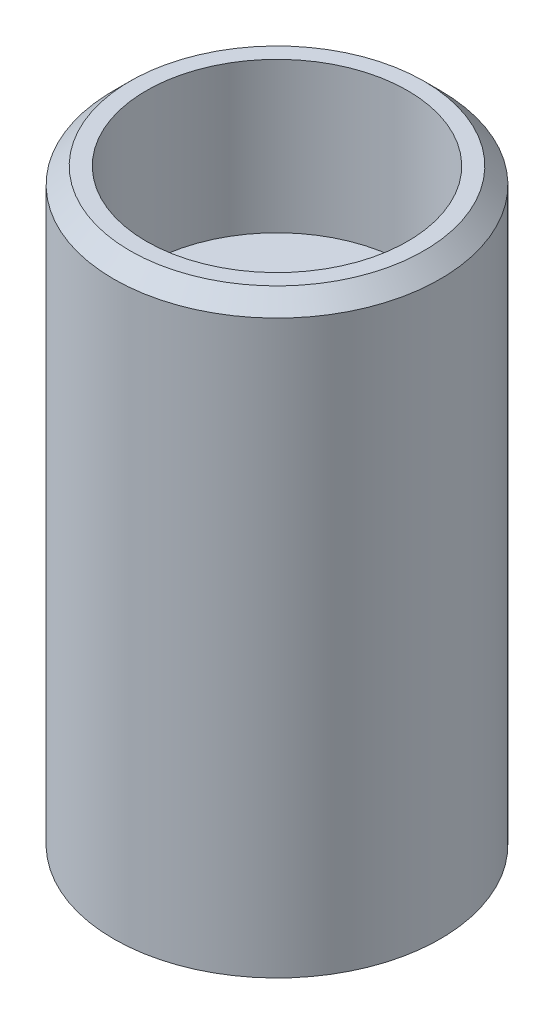
SolidWorks part; units mm, degrees
ref_plane "Front Plane" through (0, 0, 0) normal (0, 0, 1) x (1, 0, 0)
ref_plane "Top Plane" through (0, 0, 0) normal (0, 1, 0) x (1, 0, 0)
ref_plane "Right Plane" through (0, 0, 0) normal (1, 0, 0) x (0, 0, -1)
sketch "Sketch1" plane through (0, 0, 0) normal (0, 1, 0) x (1, 0, 0)
  circle A0 centre (0, 0) radius 5
  dimension "D1" = 10
extrude "Boss-Extrude1" add sketch "Sketch1" along normal blind 18
hole_wizard "Hole wizard: socket head cap screw, type 1" positions "Sketch2" profile "Sketch3" counterbore size "M4" standard "GB" end condition through all
sketch "Sketch2" plane through (0, 18, 0) normal (0, 1, 0) x (1, 0, 0)
  point P0 (0, 0)
sketch "Sketch3" plane through (0, 18, 0) normal (1, 0, 0) x (0, 0, 1)
  line L0 (0, 0) -> (0, 18)
  line L1 (0, 18) -> (2.25, 18)
  line L3 (2.25, 18) -> (2.25, 4.6)
  line L4 (2.25, 4.6) -> (4, 4.6)
  line L5 (4, 4.6) -> (4, 0)
  line L7 (4, 0) -> (0, 0)
  line L11 (0, -6.35) -> (0, 107.95) construction
  dimension "通孔孔直径" = 4.5
  dimension "通孔孔深度" = 18
  dimension "柱形沉头孔直径" = 8
  dimension "柱形沉头孔深度" = 4.6
chamfer "Chamfer1" distance 0.5 angle 45 1 edges at (0, 18, 5)
